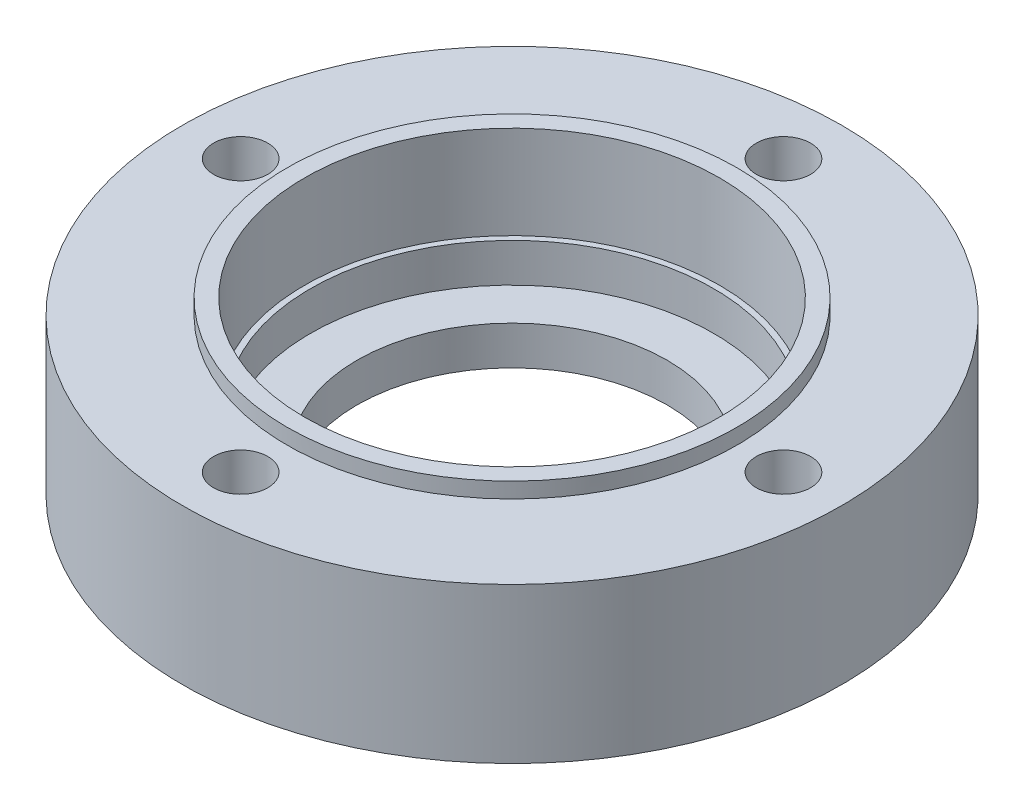
SolidWorks part; units mm, degrees
material "Q235"
ref_plane "Front Plane" through (0, 0, 0) normal (0, 0, 1) x (1, 0, 0)
ref_plane "Top Plane" through (0, 0, 0) normal (0, 1, 0) x (1, 0, 0)
ref_plane "Right Plane" through (0, 0, 0) normal (1, 0, 0) x (0, 0, -1)
sketch "Sketch1" plane through (0, 0, 0) normal (0, -1, 0) x (1, 0, 0)
  circle A0 centre (0, 0) radius 42.5
  circle A1 centre (0, 0) radius 20
  dimension "D1" = 85
  dimension "D2" = 40
extrude "Boss-Extrude1" add sketch "Sketch1" along normal blind 20
hole_wizard "M6 Clearance Hole1" positions "Sketch2" profile "Sketch3" hole size "M6" standard "GB" end condition through all
sketch "Sketch2" plane through (0, 0, 0) normal (0, 1, 0) x (1, 0, 0)
  circle A0 centre (0, 0) radius 35
  point P10 (0, 35)
  point P12 (-35, 0)
  point P14 (35, 0)
  point P16 (0, -35)
  dimension "D1" = 70
sketch "Sketch3" plane through (0, 0, 35) normal (1, 0, 0) x (0, 0, 1)
  line L0 (0, 0) -> (0, 20)
  line L1 (0, 20) -> (3.5, 20)
  line L2 (3.5, 20) -> (3.5, 0)
  line L5 (3.5, 0) -> (0, 0)
  line L11 (0, -6.35) -> (0, 107.95) construction
  dimension "通孔孔直径" = 7
  dimension "通孔孔深度" = 20
sketch "Sketch4" plane through (0, 0, 0) normal (0, 1, 0) x (1, 0, 0)
  circle A0 centre (0, 0) radius 26
  dimension "D1" = 52
extrude "Cut-Extrude1" cut sketch "Sketch4" against normal blind 15
sketch "Sketch5" plane through (0, 0, 0) normal (0, 1, 0) x (1, 0, 0)
  circle A0 centre (0, 0) radius 26.75
  circle A1 centre (0, 0) radius 29
  dimension "D1" = 53.5
  dimension "D2" = 2.25
extrude "Boss-Extrude3" add sketch "Sketch5" along normal blind 2
sketch "Sketch6" plane through (0, 2, 0) normal (0, 1, 0) x (1, 0, 0)
  circle A0 centre (0, 0) radius 26.75
  dimension "D1" = 53.5
extrude "Cut-Extrude2" cut sketch "Sketch6" against normal blind 12
sketch "Sketch7" plane through (0, -20, 0) normal (0, -1, 0) x (1, 0, 0)
  circle A0 centre (0, 35) radius 5.5
  circle A1 centre (-35, 0) radius 5.5
  circle A2 centre (0, -35) radius 5.5
  circle A3 centre (35, 0) radius 5.5
  dimension "D1" = 11
extrude "Cut-Extrude3" cut sketch "Sketch7" against normal blind 7
